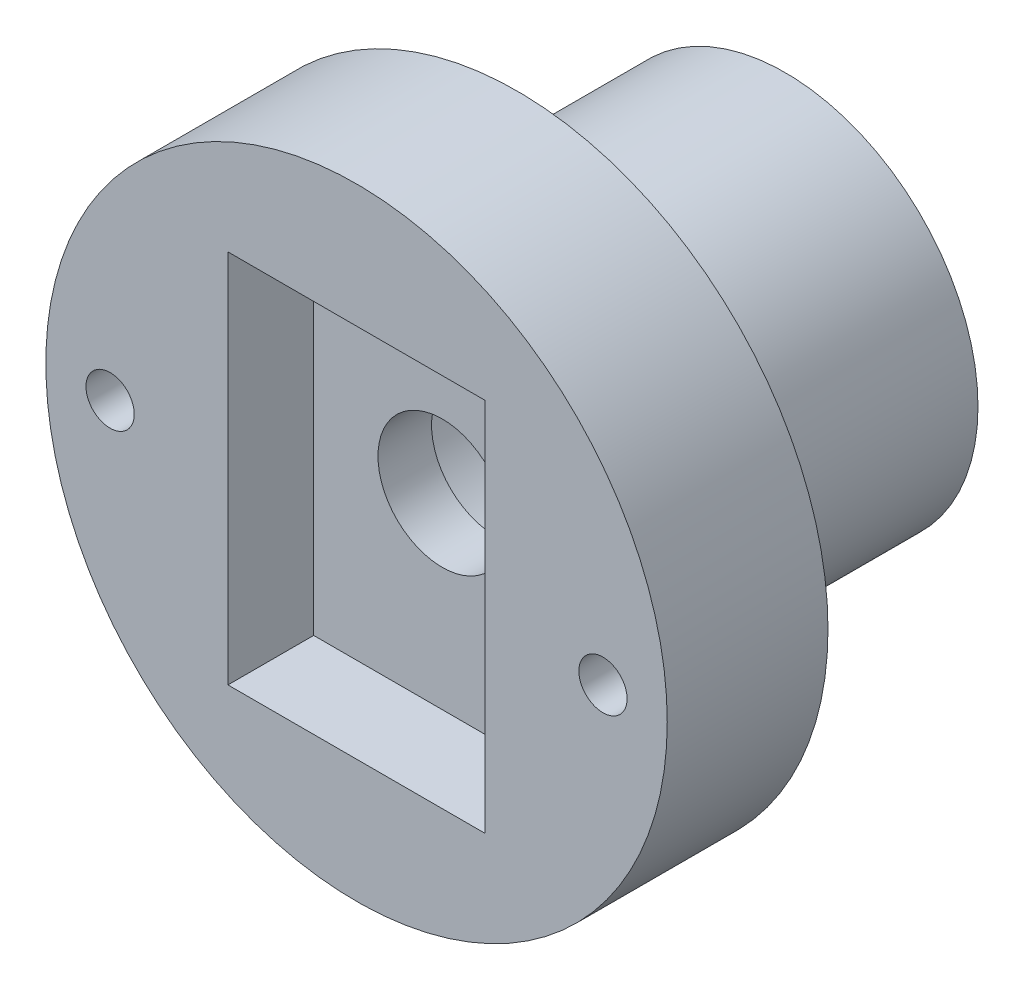
from build123d import *

# Parameters (mm, degrees)
SKETCH_1_R                = 18
SKETCH_1_R_2              = 11
EXTRUDE_1_DEPTH           = 25
SKETCH_2_R                = 29
SKETCH_2_R_2              = 11
EXTRUDE_2_DEPTH           = 15
HOLE_WIZARD_1_D           = 4.5
HOLE_WIZARD_1_CBORE_D     = 8
HOLE_WIZARD_1_CBORE_DEPTH = 4.6
SKETCH_6_W                = 24
SKETCH_6_H                = 35
CUT_EXTRUDE_1_DEPTH       = 8
EXTRUDE_START             = -5
SKETCH_7_R                = 11
SKETCH_7_R_2              = 6
EXTRUDE_3_DEPTH           = 5


with BuildPart() as part:
    # 草图1 → 凸台-拉伸1 (new body)
    with BuildSketch(Plane.XY):
        Circle(SKETCH_1_R)
        Circle(SKETCH_1_R_2, mode=Mode.SUBTRACT)
    extrude(amount=EXTRUDE_1_DEPTH)

    # 草图2 → 凸台-拉伸2 (add)
    with BuildSketch(Plane.XY.offset(25)):
        Circle(SKETCH_2_R)
        Circle(SKETCH_2_R_2, mode=Mode.SUBTRACT)
    extrude(amount=EXTRUDE_2_DEPTH)

    # 打孔尺寸根据内六角圆柱头螺钉的类型1 (through all)
    with Locations(Plane(origin=(0, 0, 25), x_dir=(-1, 0, 0), z_dir=(0, 0, -1))):
        with Locations((-23, 0), (23, 0)):
            CounterBoreHole(HOLE_WIZARD_1_D / 2, HOLE_WIZARD_1_CBORE_D / 2, HOLE_WIZARD_1_CBORE_DEPTH)

    # 草图6 → 切除-拉伸1 (cut)
    with BuildSketch(Plane.XY.offset(40)):
        Rectangle(SKETCH_6_W, SKETCH_6_H)
    extrude(amount=-CUT_EXTRUDE_1_DEPTH, mode=Mode.SUBTRACT)

    # 草图7 → 凸台-拉伸3 (add)
    with BuildSketch(Plane.XY.offset(32).offset(EXTRUDE_START)):
        Circle(SKETCH_7_R)
        Circle(SKETCH_7_R_2, mode=Mode.SUBTRACT)
    extrude(amount=EXTRUDE_3_DEPTH)


solid = part.part
